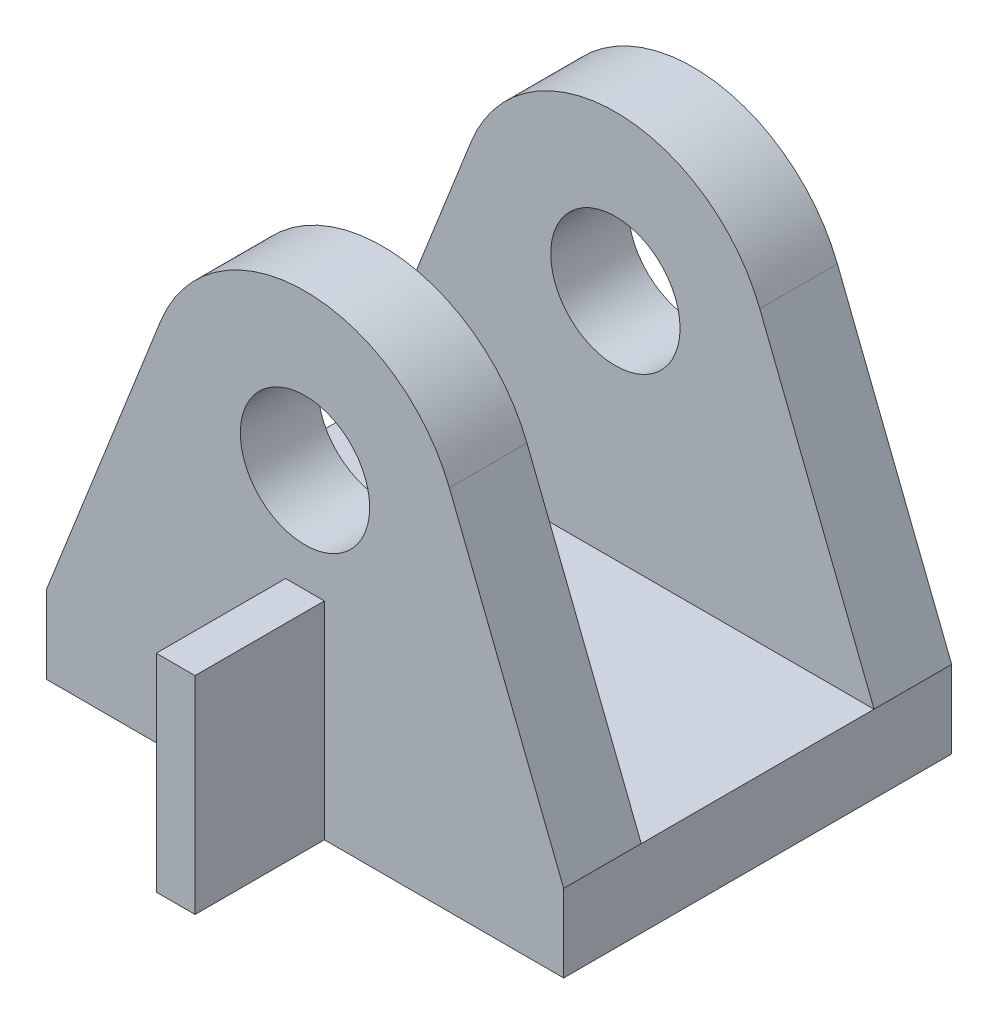
SolidWorks part; units mm, degrees
ref_plane "Front Plane" through (0, 0, 0) normal (0, 0, 1) x (1, 0, 0)
ref_plane "Top Plane" through (0, 0, 0) normal (0, 1, 0) x (1, 0, 0)
ref_plane "Right Plane" through (0, 0, 0) normal (1, 0, 0) x (0, 0, -1)
sketch "Sketch 1" plane through (0, 0, 0) normal (0, 1, 0) x (1, 0, 0)
  line L1 (-100, -75) -> (100, -75)
  line L2 (-100, -75) -> (-100, 75)
  line L3 (-100, 75) -> (100, 75)
  line L4 (100, -75) -> (100, 75)
  line L5 (-100, -75) -> (100, 75) construction
  line L6 (-100, 75) -> (100, -75) construction
  point P0 (0, 0)
  dimension "D1" = 200
  dimension "D2" = 150
extrude "Boss-Extrude 1" add sketch "Sketch 1" along normal blind 30
sketch "Sketch 2" plane through (0, 0, 75) normal (0, 0, 1) x (1, 0, 0)
  line L0 (0, -7.9075) -> (0, 168.2922) construction
  line L1 (-100, 0) -> (100, 0) construction
  line L2 (-55.8147, 142.0163) -> (-100, 30)
  line L3 (-100, 30) -> (100, 30) construction
  line L4 (-100, 30) -> (-100, 0) construction
  line L5 (-100, 30) -> (100, 30)
  line L6 (55.8147, 142.0163) -> (100, 30)
  circle A0 centre (0, 120) radius 25
  arc A1 (55.8147, 142.0163) -> (-55.8147, 142.0163) centre (0, 120) ccw
  point P17 (0, 30)
  dimension "D1" = 50
  dimension "D2" = 120
  dimension "D3" = 60
extrude "Boss-Extrude 2" add sketch "Sketch 2" against normal blind 30
sketch "Sketch 4" plane through (0, 0, 75) normal (0, 0, 1) x (1, 0, 0)
  line L0 (0, -12.2336) -> (0, 150.8827) construction
  line L1 (-100, 0) -> (100, 0) construction
  line L2 (-7.5, 80) -> (7.5, 80)
  line L3 (-7.5, 80) -> (-7.5, 0)
  line L4 (-7.5, 0) -> (7.5, 0)
  line L5 (7.5, 80) -> (7.5, 0)
  line L6 (-7.5, 80) -> (7.5, 0) construction
  line L7 (-7.5, 0) -> (7.5, 80) construction
  point P3 (0, 40)
  dimension "15" = 15
  dimension "D2" = 80
extrude "Boss-Extrude 3" add sketch "Sketch 4" along normal blind 50
mirror "Mirror 1" about plane through (0, 0, 0) normal (0, 0, 1) of "Boss-Extrude 3", "Boss-Extrude 2"
